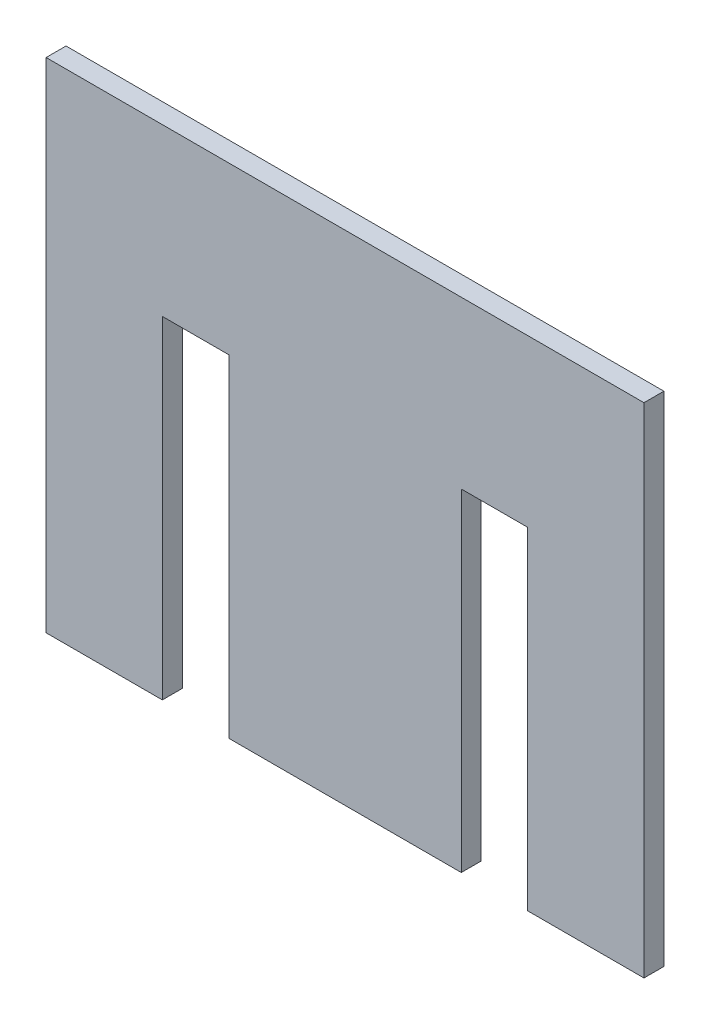
SolidWorks part; units mm, degrees
ref_plane "前视基准面" through (0, 0, 0) normal (0, 0, 1) x (1, 0, 0)
ref_plane "上视基准面" through (0, 0, 0) normal (0, 1, 0) x (1, 0, 0)
ref_plane "右视基准面" through (0, 0, 0) normal (1, 0, 0) x (0, 0, -1)
sketch "草图1" plane through (0, 0, 0) normal (0, 0, 1) x (1, 0, 0)
  line L1 (-90, -75) -> (90, -75)
  line L2 (-90, -75) -> (-90, 75)
  line L3 (-90, 75) -> (90, 75)
  line L4 (90, -75) -> (90, 75)
  line L5 (-90, -75) -> (90, 75) construction
  line L6 (-90, 75) -> (90, -75) construction
  point P0 (0, 0)
  dimension "D1" = 180
  dimension "D2" = 150
extrude "凸台-拉伸1" add sketch "草图1" along normal blind 6
sketch "草图2" plane through (0, 0, 6) normal (0, 0, 1) x (1, 0, 0)
  line L0 (-90, -75) -> (90, -75) construction
  line L1 (-55, -75) -> (-35, -75)
  line L2 (-55, -75) -> (-55, 25)
  line L3 (-55, 25) -> (-35, 25)
  line L4 (-35, -75) -> (-35, 25)
  line L5 (-90, 75) -> (-90, -75) construction
  dimension "D1" = 20
  dimension "D2" = 100
  dimension "D3" = 35
extrude "切除-拉伸1" cut sketch "草图2" against normal up to next
mirror "镜向1" about plane through (0, 0, 0) normal (1, 0, 0) of "切除-拉伸1"
